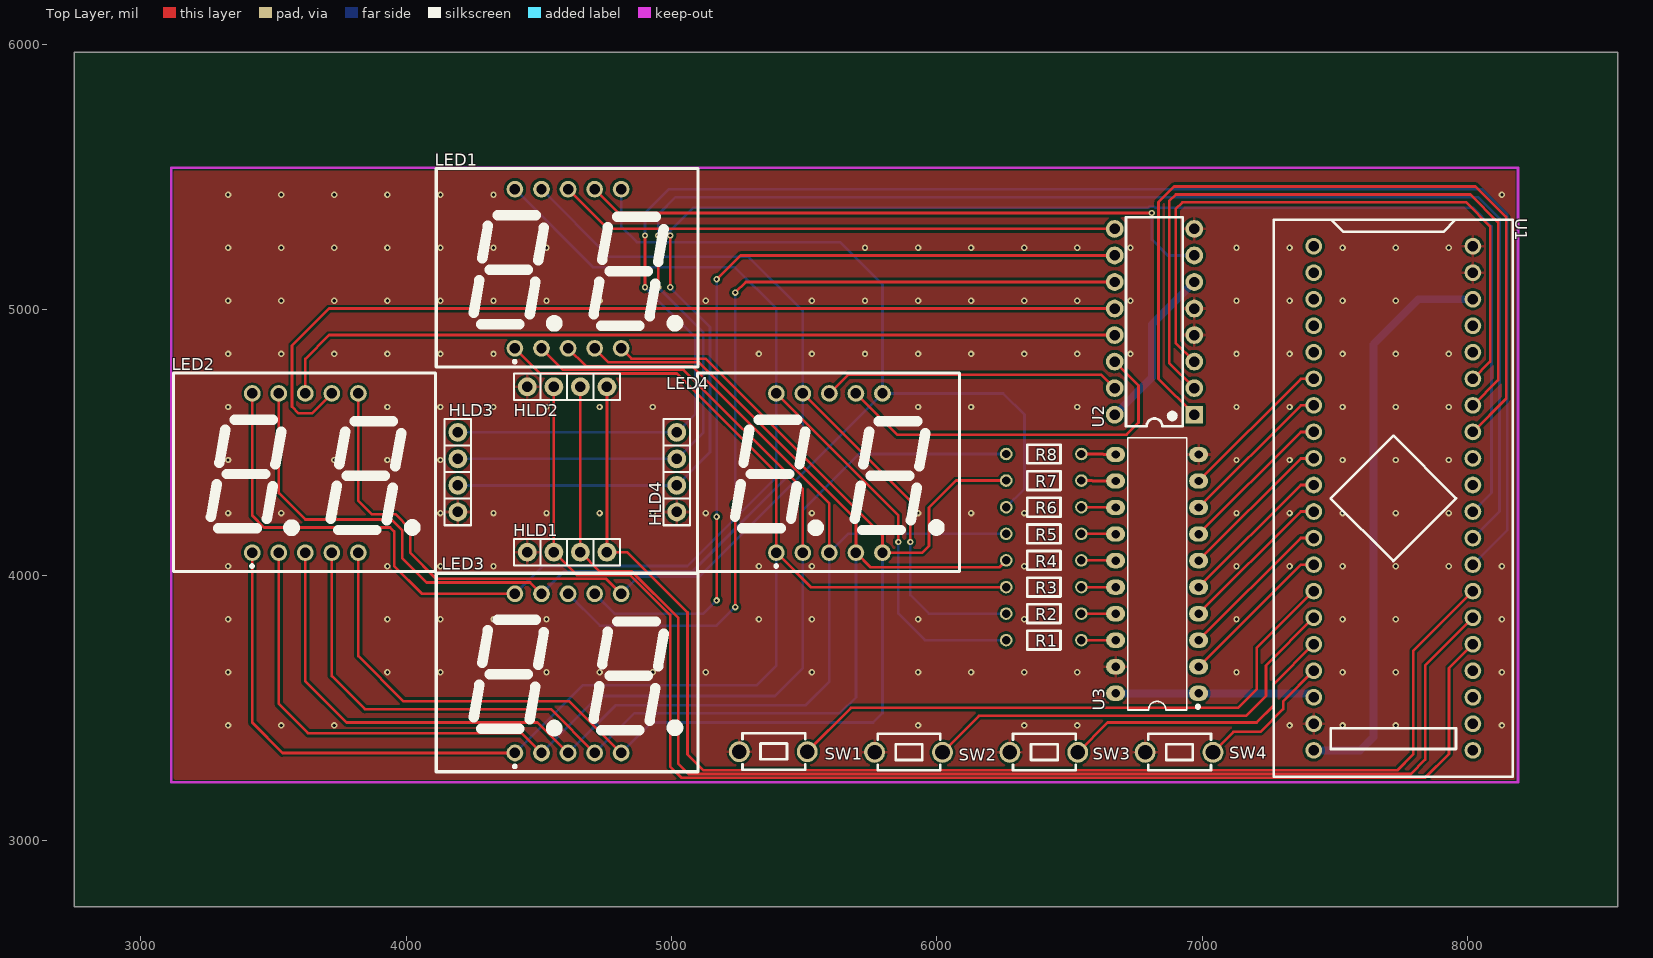
[diagram p0: Top Layer view]
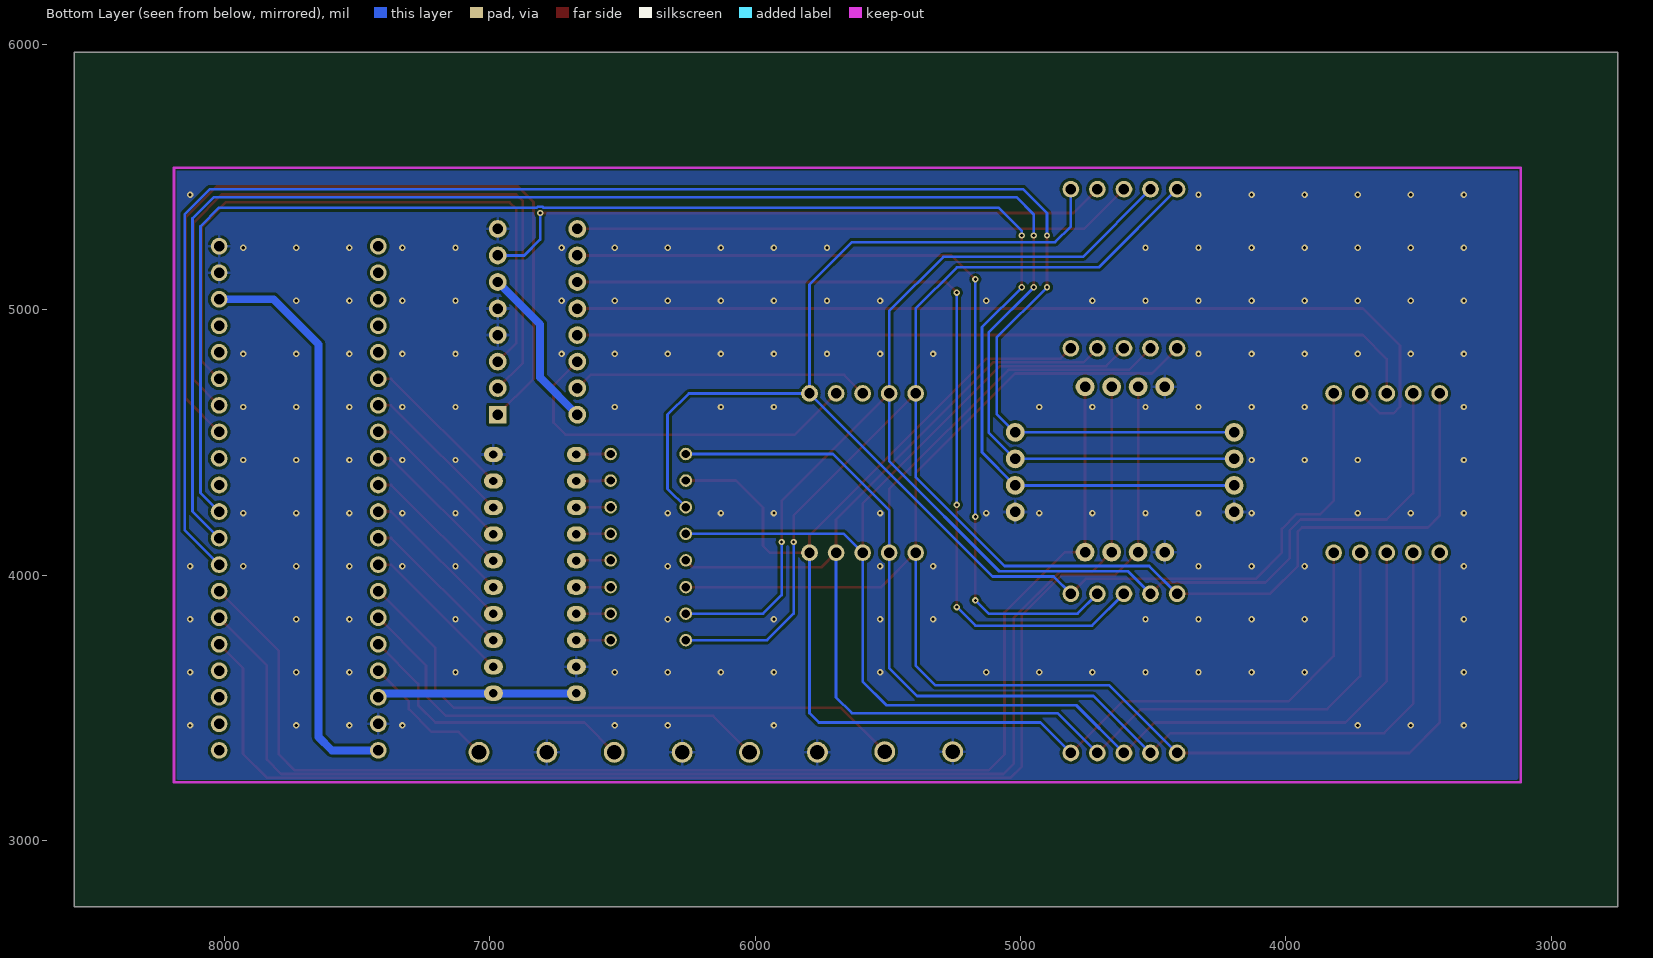
[diagram p1: Bottom Layer view, seen from below]
# Altium PCB MISC51569.pcbdoc
Units mil, origin at the board's own origin, x right, y up, seen from the top; angles counter-clockwise.
Board outline 5815 x 3220 mil, 2 copper layers (Top Layer, Bottom Layer), stack 62.206 mil thick; 23 components, 48 nets, 156 pads, 174 vias.

## Layer stack, top to bottom
Top Solder Mask Layer: solder mask 0.394, Dk 3.3
Top Layer: signal copper 1.379
Dielectric1: surface 59.449, FR4, Dk 4.5
Bottom Layer: signal copper 1.378
Bottom Solder Mask Layer: solder mask 0.394, Dk 3.3

## Board outline
8565,2750 2750,2750 2750,5970 8565,5970

## Design rules (kind name [scope] priority, off if disabled: settings)
BoardOutlineClearance copperThickness2oz_1 [All] p2 off: genericclearance=7.99 ignorepadtopadclearanceinfootprint=FALSE except(0: Arc-SplitContinuation Track-SplitContinuation SMDPad-SplitContinuation THPad-SplitContinuation Via-SplitContinuation Fill-SplitContinuation Region-SplitContinuation Poly-SplitContinuation Text-SplitContinuation Hole-SplitContinuation; 5.98: Arc-CutoutEdge SMDPad-CutoutEdge THPad-CutoutEdge Via-CutoutEdge Fill-CutoutEdge Region-CutoutEdge Text-CutoutEdge; 6.93: Hole-OutlineEdge Hole-CutoutEdge; 10: Poly-OutlineEdge Poly-CutoutEdge; 11.81: Arc-OutlineEdge Track-OutlineEdge SMDPad-OutlineEdge THPad-OutlineEdge Via-OutlineEdge Fill-OutlineEdge Region-OutlineEdge Text-OutlineEdge Track-CutoutEdge)
BoardOutlineClearance copperThickness1oz_1 [All] p4: genericclearance=4.02 ignorepadtopadclearanceinfootprint=FALSE except(0: Arc-SplitContinuation Track-SplitContinuation SMDPad-SplitContinuation THPad-SplitContinuation Via-SplitContinuation Fill-SplitContinuation Region-SplitContinuation Poly-SplitContinuation Text-SplitContinuation Hole-SplitContinuation; 6: SMDPad-CutoutEdge THPad-CutoutEdge Via-CutoutEdge Fill-CutoutEdge Region-CutoutEdge Text-CutoutEdge; 6.93: Hole-OutlineEdge Hole-CutoutEdge; 10: Poly-OutlineEdge Poly-CutoutEdge; 11.8: Arc-OutlineEdge Track-OutlineEdge SMDPad-OutlineEdge THPad-OutlineEdge Via-OutlineEdge Fill-OutlineEdge Region-OutlineEdge Text-OutlineEdge; 11.81: Arc-CutoutEdge Track-CutoutEdge)
Clearance copperThickness2oz [All] p1 off: gap=7.99 ignorepadtopadclearanceinfootprint=FALSE except(5.98: SMDPad-Track SMDPad-SMDPad THPad-Track SMDPad-THPad THPad-THPad Track-Via SMDPad-Via THPad-Via Via-Via Fill-Track Region-Track Fill-SMDPad Region-SMDPad Fill-THPad Region-THPad Fill-Via Region-Via Fill-Fill Fill-Region Region-Region Arc-Track Arc-SMDPad Arc-THPad Arc-Via Fill-Arc Region-Arc Arc-Arc Text-Track SMDPad-Text Text-THPad Text-Via Fill-Text Region-Text Arc-Text Text-Text; 6.93: Hole-Track Hole-SMDPad Hole-THPad Hole-Via Fill-Hole Region-Hole Hole-Arc Hole-Text; 10: Poly-Track Poly-SMDPad Poly-THPad Poly-Via Poly-Fill Poly-Region Poly-Poly Poly-Arc Poly-Text Poly-Hole)
Clearance copperThickness1oz [All] p3: gap=4.02 ignorepadtopadclearanceinfootprint=FALSE except(5.98: SMDPad-Track SMDPad-SMDPad THPad-Track SMDPad-THPad THPad-THPad Track-Via SMDPad-Via THPad-Via Via-Via Fill-Track Region-Track Fill-SMDPad Region-SMDPad Fill-THPad Region-THPad Fill-Via Region-Via Fill-Fill Fill-Region Region-Region; 6: Arc-Track Arc-SMDPad Arc-THPad Arc-Via Fill-Arc Region-Arc Arc-Arc Text-Track SMDPad-Text Text-THPad Text-Via Fill-Text Region-Text Arc-Text Text-Text; 6.93: Hole-Track Hole-SMDPad Hole-THPad Hole-Via Fill-Hole Region-Hole Hole-Arc Hole-Text; 10: Poly-Track Poly-SMDPad Poly-THPad Poly-Via Poly-Fill Poly-Region Poly-Poly Poly-Arc Poly-Text Poly-Hole)
DiffPairsRouting differentialPair [All] p1: maxlimit=6 minlimit=6 mostfreqgap=6 toplayer_minwidth=5 toplayer_prefwidth=10 toplayer_maxwidth=100 toplayer_mingap=6 toplayer_prefgap=6 toplayer_maxgap=6 bottomlayer_minwidth=5 bottomlayer_prefwidth=10 bottomlayer_maxwidth=100 bottomlayer_mingap=6 bottomlayer_prefgap=6 bottomlayer_maxgap=6 maxuncoupledlength=10
HoleToHoleClearance otherClearance [All] p1: gap=11.81 allowstackedmicrovias=TRUE
Length netLength [All] p1: minlimit=0 maxlimit=0
MatchedLengths netLengthTolerance [All] p1: tolerance=1000
PasteMaskExpansion pasteMaskExpansion [All] p1: expansion=0
PlaneConnect innerPlane [All] p1: planeconnectstyle=Relief reliefexpansion=20 reliefentries=4 reliefconductorwidth=10 reliefairgap=10
PolygonConnect copperRegion [(InNet('GND'))] p1: connectstyle=Relief reliefconductorwidth=10 reliefentries=4 polygonreliefangle="90 Angle" airgapwidth=10 via.connectstyle=Relief via.reliefconductorwidth=10 via.reliefentries=4 via.polygonreliefangle="90 Angle" via.airgapwidth=10
RoutingVias viaSize [All] p1: holewidth=12.01 width=24.02 viastyle="Through Hole" minholewidth=11.81 minwidth=19.68 maxholewidth=248.03 maxwidth=393.7
SolderMaskExpansion solderMaskExpansion [IsVia] p1: expansion=-1000 istentingtop=TRUE
SolderMaskExpansion solderMaskExpansion [All] p2: expansion=2 istentingtop=FALSE
Width copperThickness2oz_2 [All] p1 off: maxlimit=100 minlimit=8 preferedwidth=10
Width copperThickness1oz_2 [All] p2: maxlimit=100 minlimit=5 preferedwidth=10

## Components (designator, comment, footprint, x,y, rotation, side; value= is the part's Value field where it differs from the comment)
HLD1 "" SIP-04 4606.57,4087.12 r0 top
HLD2 "" SIP-04 4606.57,4710 r0 top
HLD3 "" SIP-04 4195,4388.4 r90 top
HLD4 "" SIP-04 5020,4388.4 r90 top
LED1 "SLR0562FW2A3BY-3.5" LED-SEG-TH_10P-L25.0-W19.0-P2.54-S15.24-BL 4610,5155 r0 top
LED2 "SLR0562FW2A3BY-3.5" LED-SEG-TH_10P-L25.0-W19.0-P2.54-S15.24-BL 3620,4385 r0 top
LED3 "SLR0562FW2A3BY-3.5" LED-SEG-TH_10P-L25.0-W19.0-P2.54-S15.24-BL 4610,3630.18 r0 top
LED4 "SLR0562FW2A3BY-3.5" LED-SEG-TH_10P-L25.0-W19.0-P2.54-S15.24-BL 5595,4385 r0 top
R1 "100R" Res_1/8W 6402.92,3757.79 r180 top
R2 "100R" Res_1/8W 6402.92,3857.79 r180 top
R3 "100R" Res_1/8W 6402.92,3957.79 r180 top
R4 "100R" Res_1/8W 6402.92,4058.27 r180 top
R5 "100R" Res_1/8W 6402.92,4158.27 r180 top
R6 "100R" Res_1/8W 6402.92,4258.76 r180 top
R7 "100R" Res_1/8W 6402.92,4359.24 r180 top
R8 "100R" Res_1/8W 6402.92,4459.24 r180 top
SW1 "" Key_TH_3.5x6x4.3 5390,3335 r180 top
SW2 "" Key_TH_3.5x6x4.3 5899.72,3332.56 r180 top
SW3 "" Key_TH_3.5x6x4.3 6409.44,3332.56 r180 top
SW4 "" Key_TH_3.5x6x4.3 6919.16,3332.56 r180 top
U1 "STM32F103C8T6-Card" CONN-TH_L53.3-W22.9_STM32F103C8T6-CARD 7720,4290 r270 top
U2 "SN74HC138NE4" PDIP-16_L19.7-W6.6-P2.54-LS7.6-BL 6820,4955 r90 top
U3 "SN74HC245N3" PDIP-20_L25.9-W6.6-P2.54-LS7.9-BL 6830,4005 r90 top

## Footprints (in the part's own frame and the unit in brackets; to place one, negate y for a bottom-side part, rotate by r counter-clockwise, add the part's x,y. Pads: shape width x height; smd on the part's side, far side on the other; paste and mask are expansions set on the pad)
CONN-TH_L53.3-W22.9_STM32F103C8T6-CARD [mm]
  round 1.6 hole 1: 1(-24.13,-7.62) 2(-21.59,-7.62) 3(-19.05,-7.62) 4(-16.51,-7.62) 5(-13.97,-7.62) 6(-11.43,-7.62) 7(-8.89,-7.62) 8(-6.35,-7.62) 9(-3.81,-7.62) 10(-1.27,-7.62) 11(1.27,-7.62) 12(3.81,-7.62) 13(6.35,-7.62) 14(8.89,-7.62) 15(11.43,-7.62) 16(13.97,-7.62) 17(16.51,-7.62) 18(19.05,-7.62) 19(21.59,-7.62) 20(24.13,-7.62) 21(24.13,7.62) 22(21.59,7.62) 23(19.05,7.62) 24(16.51,7.62) 25(13.97,7.62) 26(11.43,7.62) 27(8.89,7.62) 28(6.35,7.62) 29(3.81,7.62) 30(1.27,7.62) 31(-1.27,7.62) 32(-3.81,7.62) 33(-6.35,7.62) 34(-8.89,7.62) 35(-11.43,7.62) 36(-13.97,7.62) 37(-16.51,7.62) 38(-19.05,7.62) 39(-21.59,7.62) 40(-24.13,7.62)
  silkscreen extent -26.67,-11.43 26.67,11.43
Key_TH_3.5x6x4.3 [mil]
  round 78.7 hole 55.1 paste+0 mask+2: A(-121.44,0) B(134.46,0)
  silkscreen extent -114,-70 123,68
LED-SEG-TH_10P-L25.0-W19.0-P2.54-S15.24-BL [mm]
  round 1.6 hole 1: 1(-5.08,-7.62) 2(-2.54,-7.62) 3(0,-7.62) 4(2.54,-7.62) 5(5.08,-7.62) 6(5.08,7.62) 7(2.54,7.62) 8(0,7.62) 9(-2.54,7.62) 10(-5.08,7.62)
  silkscreen extent -12.62,-9.41 12.44,9.59
PDIP-16_L19.7-W6.6-P2.54-LS7.6-BL [mm]
  rect 1.7x1.7 hole 1: 1(-8.89,-3.81)
  round 1.7 hole 1: 2(-6.35,-3.81) 3(-3.81,-3.81) 4(-1.27,-3.81) 5(1.27,-3.81) 6(3.81,-3.81) 7(6.35,-3.81) 8(8.89,-3.81) 9(8.89,3.81) 10(6.35,3.81) 11(3.81,3.81) 12(1.27,3.81) 13(-1.27,3.81) 14(-3.81,3.81) 15(-6.35,3.81) 16(-8.89,3.81)
  silkscreen extent -10,-2.7 10,2.73
PDIP-20_L25.9-W6.6-P2.54-LS7.9-BL [mm]
  oval 1.462x1.828 hole 0.8: 1(-11.43,-3.97) 2(-8.89,-3.97) 3(-6.35,-3.97) 4(-3.81,-3.97) 5(-1.27,-3.97) 6(1.27,-3.97) 7(3.81,-3.97) 8(6.35,-3.97) 9(8.89,-3.97) 10(11.43,-3.97) 11(11.43,3.97) 12(8.89,3.97) 13(6.35,3.97) 14(3.81,3.97) 15(1.27,3.97) 16(-1.27,3.97) 17(-3.81,3.97) 18(-6.35,3.97) 19(-8.89,3.97) 20(-11.43,3.97)
  silkscreen extent -13.03,-4.05 13.03,2.83
Res_1/8W [mil]
  round 47.2 hole 31.5 paste+0 mask+2: 1(-141.7,2.48) 2(141.7,2.48)
  silkscreen extent -63,-33 63,38
SIP-04 [mm]
  round 1.8 hole 1: 1(-3.81,0) 2(-1.27,0) 3(1.27,0) 4(3.81,0)
  silkscreen extent -5.08,-1.27 5.08,1.27

## Via types
v1: diameter 24.02, hole 12, Top Layer to Bottom Layer, 174 vias

## Nets (pads, with @x,y where several pads share a name; then routed paths per layer and width w, separated by ;. In a path a pad name is that pad's centre, name@x,y a point inside that pad or via, vN(x,y) a via of type N, cw(c..) or ccw(c..) an arc to the next point about the centre after c; other vN are vias at no path point)
$1N143: R1.1 U3.18 | length 129.2
  Top Layer w10: R1.1 6673.39,3755.31 U3.18
$1N144: R2.1 U3.17 | length 129.2
  Top Layer w10: R2.1 6673.39,3855.31 U3.17
$1N145: R3.1 U3.16 | length 129.2
  Top Layer w10: R3.1 6673.39,3955.31 U3.16
$1N146: R4.1 U3.15 | length 129.4
  Top Layer w10: R4.1 6672.91,4055.79 U3.15
$1N147: R5.1 U3.14 | length 129.4
  Top Layer w10: R5.1 6672.91,4155.79 U3.14
$1N148: R6.1 U3.13 | length 129.6
  Top Layer w10: R6.1 6672.42,4256.28 U3.13
$1N149: R7.1 U3.12 | length 129.8
  Top Layer w10: R7.1 6584.54,4356.76 6586.3,4355 U3.12
$1N150: R8.1 U3.11 | length 129.8
  Top Layer w10: R8.1 6625.96,4456.76 6627.73,4455 U3.11
+5V: U1.18 U2.6 U2.16 U3.1 U3.20 | length 1376.8
  Bottom Layer w30: U2.16 6810,4745 6810,4945 U2.6 ; U3.20 U3.1 7405,3555 U1.18
A: LED1.10 LED2.10 LED3.10 LED4.10 R1.2 | length 6089.9
  Top Layer w10: LED2.10 3420,4225 3465,4180 3940,4180 3955,4165 3955,4035 4059.82,3930.18 LED3.10 ; LED4.10 5855,4225 v1(5855,4125)
  Bottom Layer w10: LED3.10 4514.82,4035 5060,4035 5395,4370 LED4.10 5395,5005 5240,5160 4705,5160 LED1.10 ; v1(5855,4125) 5855,3855 5954.69,3755.31 R1.2
B: LED1.9 LED2.9 LED3.9 LED4.9 R2.2 | length 5834.2
  Top Layer w10: LED2.9 3520,4310 3620,4210 3945,4210 3985,4170 3985,4065 4077.34,3972.66 4467.52,3972.66 LED3.9 ; LED4.9 5900,4280 v1(5900,4125)
  Bottom Layer w10: LED3.9 4594.82,4015 5080,4015 5495,4430 LED4.9 5495,4995 5290,5200 4765,5200 LED1.9 ; v1(5900,4125) 5900,3925 5969.69,3855.31 R2.2
C: LED1.1 LED2.1 LED3.1 LED4.1 R3.2 | length 5623.8
  Top Layer w10: LED2.1 3420,3445 3534.82,3330.18 LED3.1 ; LED1.1 4505,4760 5020,4760 5395,4385 LED4.1 5524.69,3955.31 R3.2
  Bottom Layer w10: LED3.1 4664.82,3585 5320,3585 5395,3660 LED4.1
D: LED1.4 LED2.4 LED3.4 LED4.4 R4.2 | length 5168.8
  Top Layer w10: LED2.4 3720,3620 3845,3495 4545.18,3495 LED3.4 ; LED1.4 4762.95,4802.05 5102.95,4802.05 5695,4210 LED4.4 5750,4030 6235.43,4030 R4.2
  Bottom Layer w10: LED3.4 4859.82,3480 5635,3480 5695,3540 LED4.4
DP: LED1.2 LED2.2 LED3.2 LED4.2 R8.2 | length 5647.5
  Top Layer w10: LED2.2 3520,3515 3630,3405 4435.18,3405 LED3.2 ; LED1.2 4590.98,4774.02 5045.98,4774.02 5495,4325 LED4.2
  Bottom Layer w10: LED3.2 4724.82,3545 5390,3545 5495,3650 LED4.2 5495,4245 5706.76,4456.76 R8.2
E: LED1.3 LED2.3 LED3.3 LED4.3 R5.2 | length 5276.4
  Top Layer w10: LED2.3 3620,3600 3775,3445 4495.18,3445 LED3.3 ; LED1.3 4676.97,4788.03 5076.97,4788.03 5595,4270 LED4.3
  Bottom Layer w10: LED3.3 4789.82,3510 5505,3510 5595,3600 LED4.3 5665.79,4155.79 R5.2
F: LED1.6 LED2.6 LED3.6 LED4.6 R6.2 | length 5461.8
  Top Layer w10: LED2.6 3820,4280 3870,4230 3960,4230 4015,4175 4015,4085 4113.32,3986.68 4753.5,3986.68 LED3.6
  Bottom Layer w10: LED3.6 4874.82,3995 5105,3995 LED4.6 ; LED1.6 4810,5315 4870,5255 5635,5255 5795,5095 LED4.6 ; R6.2 6330,4325.06 6330,4605 6250,4685 LED4.6
G: LED1.5 LED2.5 LED3.5 LED4.5 R7.2 | length 5188.9
  Top Layer w10: LED2.5 3820,3695 3990,3525 4615.18,3525 LED3.5 ; LED1.5 4848.94,4816.06 5128.94,4816.06 5795,4150 LED4.5 5945,4085 5970,4110 5970,4255 6071.76,4356.76 R7.2
  Bottom Layer w10: LED3.5 4924.82,3445 5760,3445 5795,3480 LED4.5
GND: HLD1.1 HLD2.1 HLD3.1 HLD4.1 SW1.B SW2.B SW3.B SW4.B U1.19 U1.39 U1.40 U2.4 U2.5 U2.8 U3.10 U3.19
  other v1: 3329.1,3434.1 3529.1,3434.1 3729.1,3434.1 5929.1,3434.1 6329.1,3434.1 6529.1,3434.1 7329.1,3434.1 7529.1,3434.1 7729.1,3434.1 8129.1,3434.1 3329.1,3634.1 3929.1,3634.1 4129.1,3634.1 4329.1,3634.1 4529.1,3634.1 4729.1,3634.1 4929.1,3634.1 5129.1,3634.1 5529.1,3634.1 5929.1,3634.1 6129.1,3634.1 6329.1,3634.1 6529.1,3634.1 7129.1,3634.1 7529.1,3634.1 7729.1,3634.1 8129.1,3634.1 3329.1,3834.1 3929.1,3834.1 4129.1,3834.1 4329.1,3834.1 4529.1,3834.1 5329.1,3834.1 5529.1,3834.1 5929.1,3834.1 6329.1,3834.1 7129.1,3834.1 7529.1,3834.1 7729.1,3834.1 8129.1,3834.1 3329.1,4034.1 3929.1,4034.1 4129.1,4034.1 4329.1,4034.1 5329.1,4034.1 5529.1,4034.1 6329.1,4034.1 7129.1,4034.1 7329.1,4034.1 7529.1,4034.1 7729.1,4034.1 7929.1,4034.1 8129.1,4034.1 3329.1,4234.1 3529.1,4234.1 3729.1,4234.1 4129.1,4234.1 4329.1,4234.1 4529.1,4234.1 4729.1,4234.1 4929.1,4234.1 5129.1,4234.1 5529.1,4234.1 5929.1,4234.1 6129.1,4234.1 6329.1,4234.1 7129.1,4234.1 7329.1,4234.1 7529.1,4234.1 7729.1,4234.1 7929.1,4234.1 3329.1,4434.1 3729.1,4434.1 3929.1,4434.1 4129.1,4434.1 7129.1,4434.1 7329.1,4434.1 7529.1,4434.1 7729.1,4434.1 7929.1,4434.1 3329.1,4634.1 3929.1,4634.1 4129.1,4634.1 4329.1,4634.1 4529.1,4634.1 4729.1,4634.1 4929.1,4634.1 5929.1,4634.1 6129.1,4634.1 6529.1,4634.1 7129.1,4634.1 7329.1,4634.1 7529.1,4634.1 7729.1,4634.1 7929.1,4634.1 3329.1,4834.1 3529.1,4834.1 3729.1,4834.1 3929.1,4834.1 4129.1,4834.1 4329.1,4834.1 5329.1,4834.1 5529.1,4834.1 5729.1,4834.1 5929.1,4834.1 6129.1,4834.1 6329.1,4834.1 6529.1,4834.1 6729.1,4834.1 7129.1,4834.1 7329.1,4834.1 7529.1,4834.1 7729.1,4834.1 7929.1,4834.1 3329.1,5034.1 3529.1,5034.1 3729.1,5034.1 3929.1,5034.1 4129.1,5034.1 4329.1,5034.1 4529.1,5034.1 4729.1,5034.1 5129.1,5034.1 5529.1,5034.1 5729.1,5034.1 5929.1,5034.1 6129.1,5034.1 6329.1,5034.1 6529.1,5034.1 6729.1,5034.1 7129.1,5034.1 7329.1,5034.1 7529.1,5034.1 7729.1,5034.1 3329.1,5234.1 3529.1,5234.1 3729.1,5234.1 3929.1,5234.1 4129.1,5234.1 4329.1,5234.1 4529.1,5234.1 5729.1,5234.1 5929.1,5234.1 6129.1,5234.1 6329.1,5234.1 6529.1,5234.1 6729.1,5234.1 7129.1,5234.1 7329.1,5234.1 7529.1,5234.1 7729.1,5234.1 7929.1,5234.1 3329.1,5434.1 3529.1,5434.1 3729.1,5434.1 3929.1,5434.1 4129.1,5434.1 4329.1,5434.1 8129.1,5434.1
LED1: LED4.8 U2.15 | length 1124.7
  Top Layer w10: LED4.8 5665,4755 6620,4755 U2.15
LED2: LED4.7 U2.14 | length 1415.1
  Top Layer w10: LED4.7 5850,4530 6715,4530 6760,4575 6760,4715 U2.14
LED3: LED2.8 U2.13 | length 3217.3
  Top Layer w10: LED2.8 3620,4815 3710,4905 U2.13
LED4: LED2.7 U2.12 | length 3579.4
  Top Layer w10: LED2.7 3645,4610 3595,4610 3570,4635 3570,4865 3710,5005 U2.12
LED5: LED3.8 U2.11 | length 3340.3
  Top Layer w10: v1(5240,3880) v1(5240,4265) ; v1(5240,5065) 5280,5105 U2.11
  Bottom Layer w10: LED3.8 4730.18,3810 5170,3810 v1(5240,3880) ; v1(5240,4265) v1(5240,5065)
LED6: LED3.7 U2.10 | length 3259.1
  Top Layer w10: v1(5170,3905) v1(5170,4220) ; v1(5170,5115) 5260,5205 U2.10
  Bottom Layer w10: LED3.7 4785.18,3855 5120,3855 v1(5170,3905) ; v1(5170,4220) v1(5170,5115)
LED7: LED1.8 U2.9 | length 2122.1
  Top Layer w10: LED1.8 4760,5305 U2.9
LED8: LED1.7 U2.7 | length 2422.1
  Top Layer w10: LED1.7 4800,5365 v1(6810,5365)
  Bottom Layer w10: v1(6810,5365) 6810,5265 6870,5205 U2.7
PA0: HLD1.2 HLD2.2 U1.25 | length 5170.2
  Top Layer w10: HLD2.2 HLD1.2 4643,4000.69 4844.31,4000.69 4995,3850 4995,3280 5038.2,3236.8 7840,3236.8 7930,3326.8 7930,3650 U1.25
PA1: HLD1.3 HLD2.3 U1.26 | length 5106.8
  Top Layer w10: HLD2.3 HLD1.3 4728.99,4014.71 4850.11,4014.71 5025,3839.82 5025,3290 5064.18,3250.82 7785.82,3250.82 7840,3305 7840,3660 U1.26
PA2: HLD1.4 HLD2.4 U1.27 | length 5048.4
  Top Layer w10: HLD2.4 HLD1.4 4832.88,4087.12 5060,3860 5060,3325 5120.17,3264.83 7734.83,3264.83 7795,3325 7795,3715 U1.27
PA3: HLD3.4 HLD4.4 U1.28 | length 6459.8
  Top Layer w10: v1(4900,5085) v1(4900,5280)
  Bottom Layer w10: HLD3.4 HLD4.4 5090,4608.4 5090,4895 v1(4900,5085) ; v1(4900,5280) 4900,5365 4990,5455 8055,5455 8150,5360 8150,4170 U1.28
PA4: HLD3.3 HLD4.3 U1.29 | length 6334.9
  Top Layer w10: v1(4950,5085) v1(4950,5280)
  Bottom Layer w10: HLD3.3 HLD4.3 5120,4538.4 5120,4915 v1(4950,5085) ; v1(4950,5280) 4950,5360 5015,5425 8040,5425 8120,5345 8120,4240 U1.29
PA5: HLD3.2 HLD4.2 U1.30 | length 6164.7
  Top Layer w10: v1(4995,5085) v1(4995,5280)
  Bottom Layer w10: HLD3.2 HLD4.2 5145,4463.4 5145,4935 v1(4995,5085) ; v1(4995,5280) 4995,5297.41 5082.59,5385 6797.48,5385 6800.48,5387.99 6819.52,5387.99 6822.52,5385 8020,5385 8090,5315 8090,4310 U1.30
PB0: U1.33 U2.1 | length 3101
  Top Layer w10: U2.1 6835,4740 6835,5406.33 6893.67,5465 8030,5465 8145,5350 8145,4665 U1.33
PB1: U1.34 U2.2 | length 2767.2
  Top Layer w10: U2.2 6875,4800 6875,5409.46 6900.54,5435 8010,5435 8115,5330 8115,4735 U1.34
PB2: U1.35 U2.3 | length 2438.6
  Top Layer w10: U2.3 6900,4875 6900,5380 6925,5405 7995,5405 8085,5315 8085,4805 U1.35
PB6: SW1.A U1.14 | length 2250
  Top Layer w10: SW1.A 5676.44,3500 7135,3500 7205,3570 7205,3725 U1.14
PB7: SW2.A U1.15 | length 1676.4
  Top Layer w10: SW2.A 6158.6,3470 7165,3470 7240,3545 7240,3660 U1.15
PB8: SW3.A U1.16 | length 1104.7
  Top Layer w10: SW3.A 6643.32,3445 7205,3445 7270,3510 7270,3590 U1.16
PB9: SW4.A U1.17 | length 524.3
  Top Layer w10: SW4.A 7118.05,3410 7220,3410 7305,3495 7305,3525 U1.17
PC0: U1.13 U3.2 | length 593.2
  Top Layer w10: U3.2 7371.3,4040 U1.13
PC1: U1.12 U3.3 | length 593.2
  Top Layer w10: U3.3 7371.3,4140 U1.12
PC2: U1.11 U3.4 | length 593.2
  Top Layer w10: U3.4 7371.3,4240 U1.11
PC3: U1.10 U3.5 | length 593.2
  Top Layer w10: U3.5 7371.3,4340 U1.10
PC4: U1.9 U3.6 | length 593.2
  Top Layer w10: U3.6 7371.3,4440 U1.9
PC5: U1.8 U3.7 | length 593.2
  Top Layer w10: U3.7 7371.3,4540 U1.8
PC6: U1.7 U3.8 | length 593.2
  Top Layer w10: U3.8 7371.3,4640 U1.7
PC7: U1.6 U3.9 | length 593.2
  Top Layer w10: U3.9 7371.3,4740 U1.6
VCC: U1.20 U1.38 | length 2171.1
  Bottom Layer w30: U1.20 7595,3340 7645,3390 7645,4870 7815,5040 U1.38
pads on no net: U1.1 U1.2 U1.3 U1.4 U1.5 U1.21 U1.22 U1.23 U1.24 U1.31 U1.32 U1.36 U1.37

## Polygon pours and split planes (outlines as drawn)
GND on Top Layer (solid, remove dead copper, pour order 0): 3060,5700 3060,3000 8315,3000 8315,5700
GND on Bottom Layer (solid, remove dead copper, pour order 2): 3000,5720 3000,3065 8240,3065 8240,5720

## Keep-outs
Board Outline Layer:
  lines w10: 3115,3220 3115,5535 8190,5535 8190,3220 3115,3220